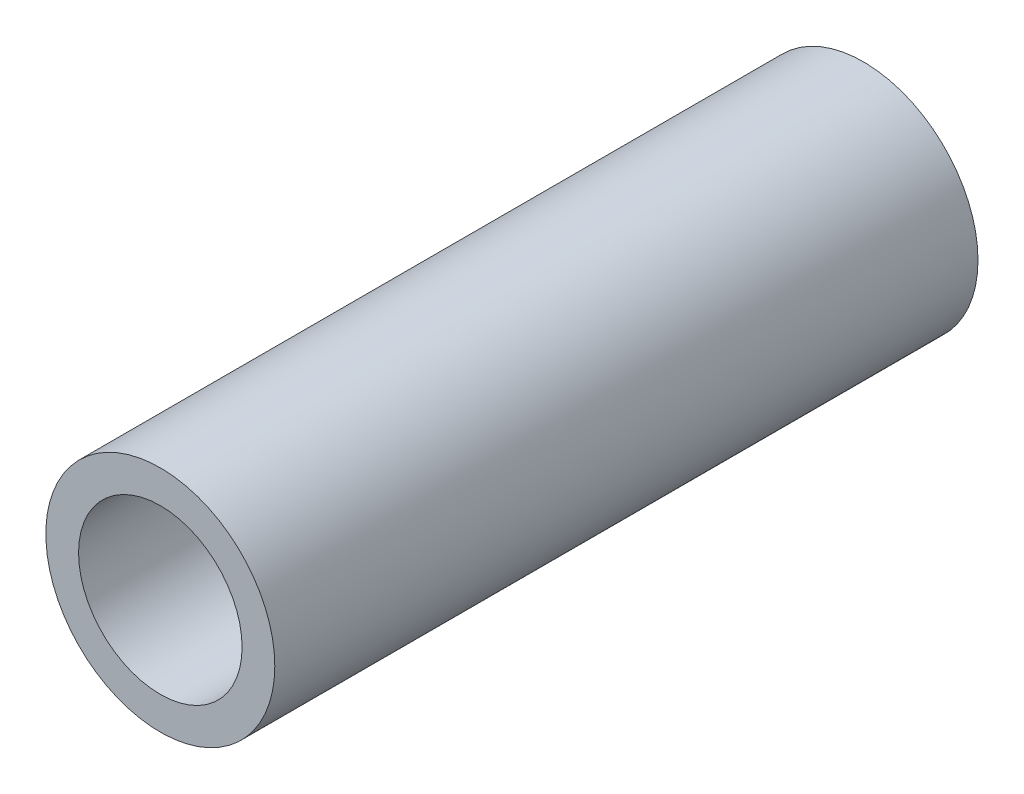
SolidWorks part; units mm, degrees
ref_plane "前视基准面" through (0, 0, 0) normal (0, 0, 1) x (1, 0, 0)
ref_plane "上视基准面" through (0, 0, 0) normal (0, 1, 0) x (1, 0, 0)
ref_plane "右视基准面" through (0, 0, 0) normal (1, 0, 0) x (0, 0, -1)
sketch "草图1" plane through (0, 0, 0) normal (0, 0, 1) x (1, 0, 0)
  circle A0 centre (0, 0) radius 5
  circle A1 centre (0, 0) radius 7
  dimension "D1" = 10
  dimension "D2" = 14
extrude "凸台-拉伸1" add sketch "草图1" along normal blind 43
